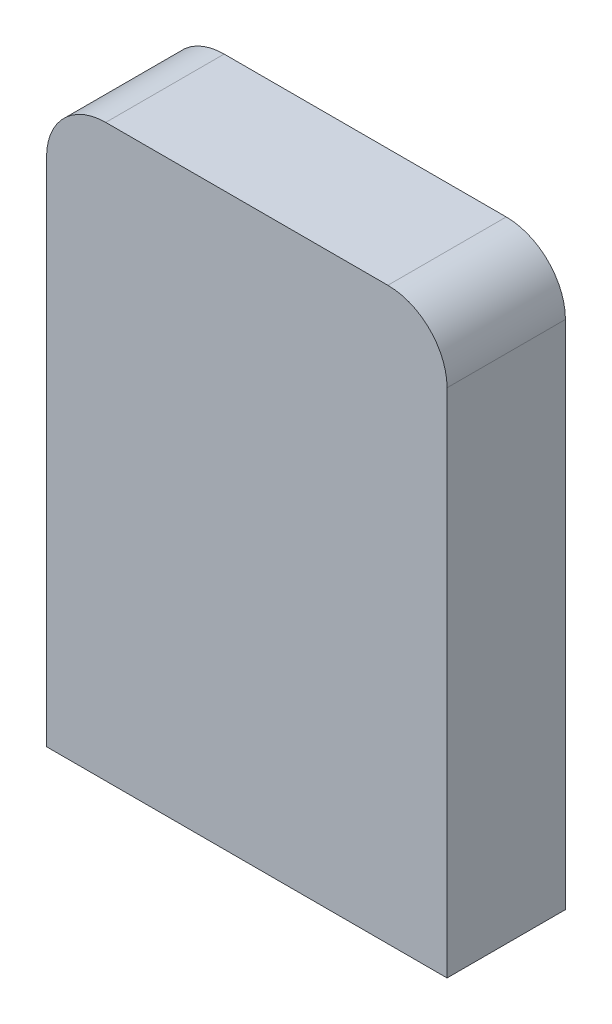
from build123d import *

# Parameters (mm, degrees)
BOSS_EXTRUDE1_DEPTH = 40
SHELL1_T            = -5


with BuildPart() as part:
    # Sketch1 → Boss-Extrude1 (new body)
    with BuildSketch(Plane.XY):
        with BuildLine():
            Line((-11.59263729, -51.941945741), (92.170688637, -51.941945741))
            Line((92.170688637, -51.941945741), (123.739238561, -51.941945741))
            Line((123.739238561, -51.941945741), (123.739238561, 120.781051565))
            ThreePointArc((123.739238561, 120.781051565), (117.881374185, 134.923187188), (103.739238561, 140.781051565))
            Line((103.739238561, 140.781051565), (8.40736271, 140.781051565))
            ThreePointArc((8.40736271, 140.781051565), (-5.734772914, 134.923187188), (-11.59263729, 120.781051565))
            Line((-11.59263729, 120.781051565), (-11.59263729, -51.941945741))
        make_face()
    extrude(amount=BOSS_EXTRUDE1_DEPTH)

    # Shell1
    shell1_openings = [part.faces().sort_by_distance(p)[0] for p in [
        (56.073300636, 43.810653181, 0),
    ]]
    offset(amount=SHELL1_T, openings=shell1_openings, kind=Kind.INTERSECTION)


solid = part.part
